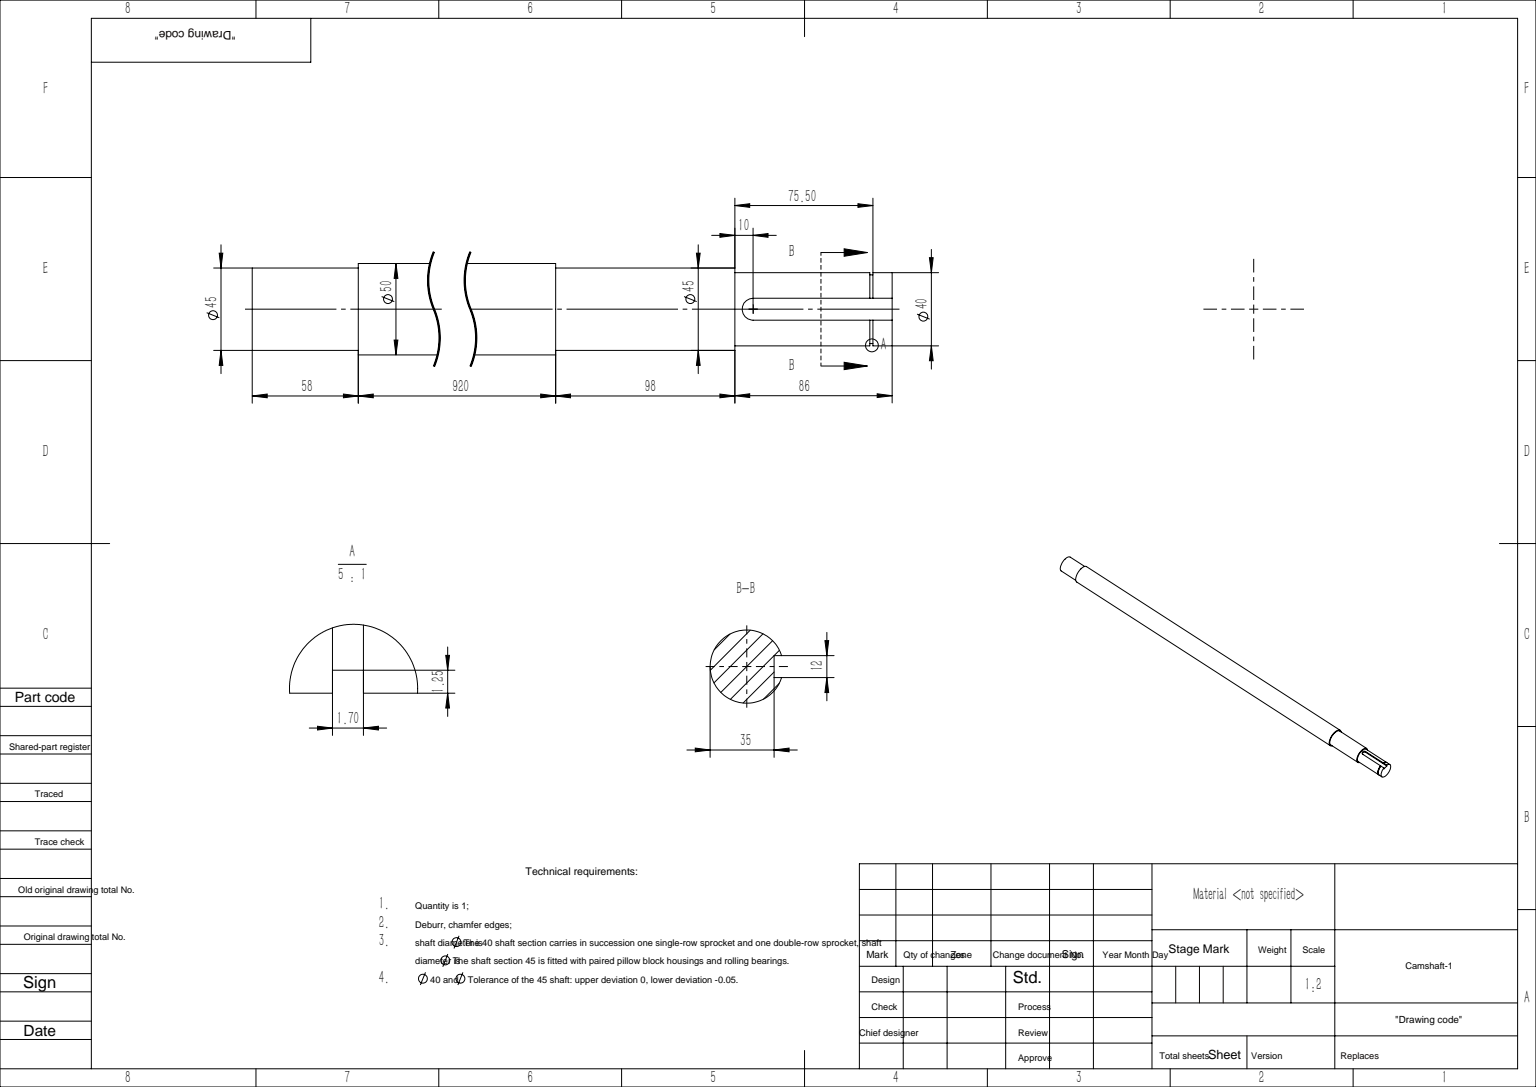
from build123d import *

# Parameters (mm, degrees)
CUT_EXTRUDE_1_DEPTH = 5
SKETCH_3_R          = 20
SKETCH_3_R_2        = 18.75
CUT_EXTRUDE_2_DEPTH = 1.7


with BuildPart() as part:
    # 草图1 → 旋转1 (revolve)
    with BuildSketch(Plane.XY):
        Polygon((0, 0), (0, 22.5), (58, 22.5), (58, 25), (978, 25), (978, 22.5), (1076, 22.5), (1076, 20), (1162, 20), (1162, 0), align=None)
    revolve(axis=Axis((1162, 0, 0), (-1, 0, 0)))

    # 草图2 → 切除-拉伸1 (cut)
    with BuildSketch(Plane(origin=(0, 20, 0), x_dir=(1, 0, 0), z_dir=(0, 1, 0))):
        with BuildLine():
            Line((1086, 6), (1172, 6))
            Line((1172, 6), (1172, -6))
            Line((1172, -6), (1086, -6))
            ThreePointArc((1086, -6), (1080, 0), (1086, 6))
        make_face()
    extrude(amount=-CUT_EXTRUDE_1_DEPTH, mode=Mode.SUBTRACT)

    # 草图3 → 切除-拉伸2 (cut)
    with BuildSketch(Plane(origin=(1151.5, 0, 0), x_dir=(0, 0, -1), z_dir=(1, 0, 0))):
        with Locations(Location((0, 0, 0), (0, 0, 90))):
            Circle(SKETCH_3_R)
        Circle(SKETCH_3_R_2, mode=Mode.SUBTRACT)
    extrude(amount=-CUT_EXTRUDE_2_DEPTH, mode=Mode.SUBTRACT)


solid = part.part
